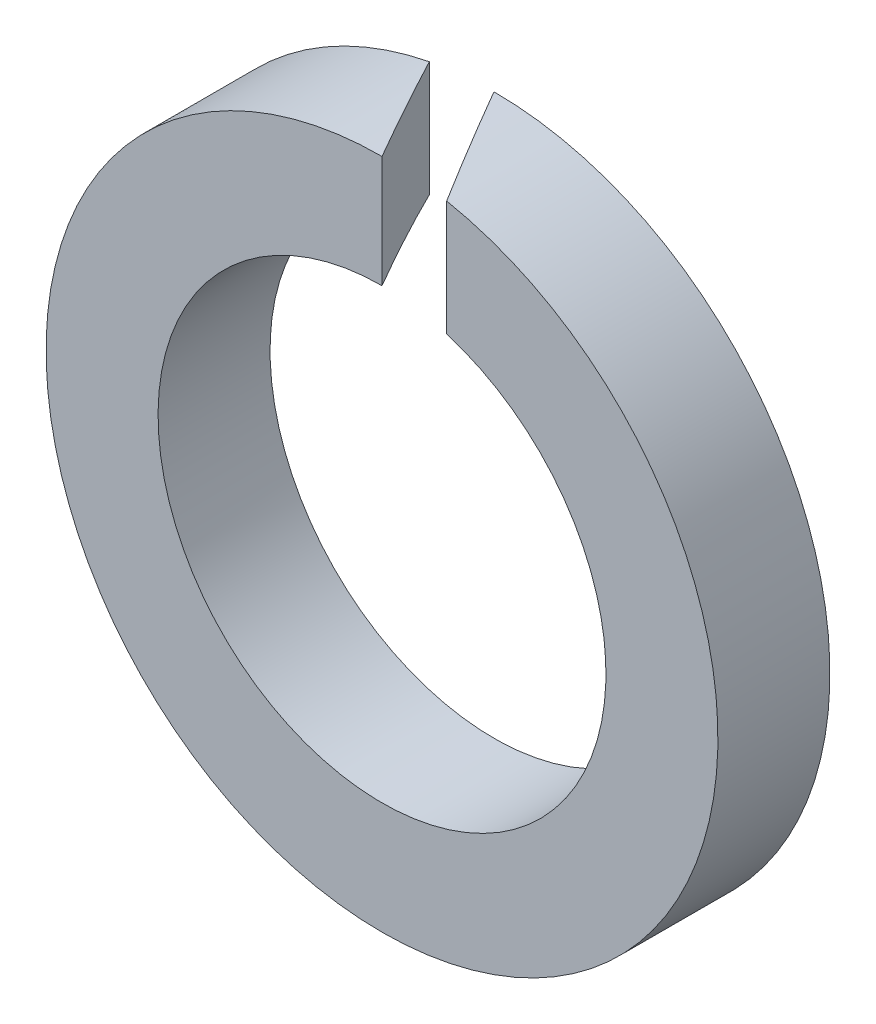
SolidWorks part; units mm, degrees
material "316L"
ref_plane "Front" through (0, 0, 0) normal (0, 0, 1) x (1, 0, 0)
ref_plane "Top" through (0, 0, 0) normal (0, 1, 0) x (1, 0, 0)
ref_plane "Right" through (0, 0, 0) normal (1, 0, 0) x (0, 0, -1)
sketch "Sketch1" plane through (0, 0, 0) normal (0, 0, 1) x (1, 0, 0)
  circle A0 centre (0, 0) radius 2.2
  circle A1 centre (0, 0) radius 3.3
  dimension "d" = 4.4
  dimension "b" = 1.1
extrude "Base-Extrude" add sketch "Sketch1" against normal blind 1.1
sketch "Sketch2" plane through (0, 0, 0) normal (0, 1, 0) x (1, 0, 0)
  line L0 (0, 1.1) -> (0.6351, 0)
  line L1 (0.6351, 0) -> (0, 0)
  line L3 (0, 0) -> (-0.6351, 1.1)
  line L5 (-0.6351, 1.1) -> (0, 1.1)
  line L7 (3.3, 1.1) -> (-3.3, 1.1) construction
  dimension "m" = 0.55
extrude "Cut-Extrude1" cut sketch "Sketch2" along normal through all
